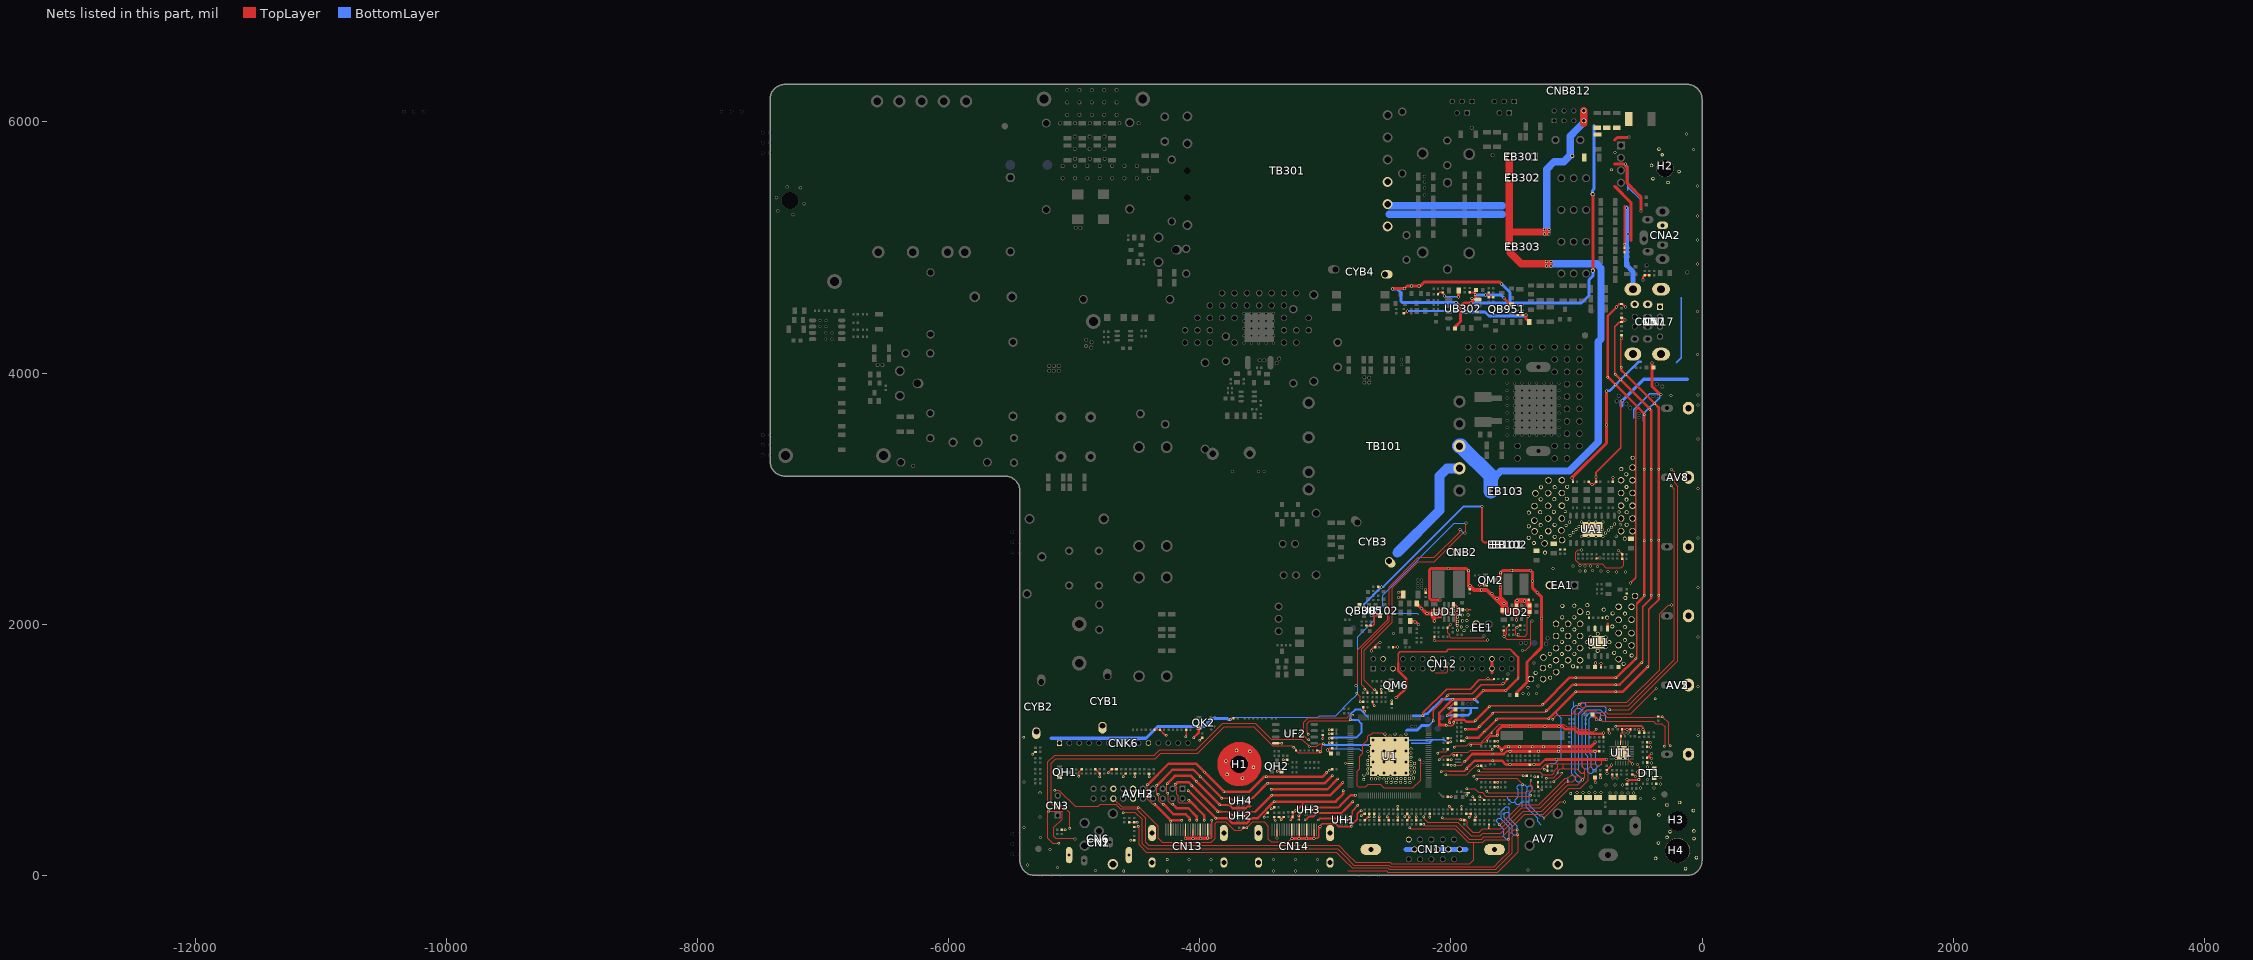
[diagram p0: the nets of this part, all layers, seen from the top]
# Altium PCB MISC84277.PcbDoc (part 9 of 15)
Units mil, origin at the board's own origin, x right, y up, seen from the top; angles counter-clockwise.
Board outline 7422.08 x 6299.21 mil, 2 copper layers (TopLayer, BottomLayer), stack 61.855 mil thick; 709 components, 395 nets, 2812 pads, 811 vias.

## Via types
v1: diameter 23.62, hole 15.75, TopLayer to BottomLayer, tented both sides, 437 vias
v2: diameter 19.68, hole 11.81, TopLayer to BottomLayer, tented both sides, 353 vias
v3: diameter 31.5, hole 23.62, TopLayer to BottomLayer, tented both sides, 16 vias
v4: diameter 31.5, hole 19.68, TopLayer to BottomLayer, tented both sides, 4 vias
v5: diameter 17.72, hole 9.84, TopLayer to BottomLayer, tented both sides, 1 vias

## Nets (pads, with @x,y where several pads share a name; then routed paths per layer and width w, separated by ;. In a path a pad name is that pad's centre, name@x,y a point inside that pad or via, vN(x,y) a via of type N, cw(c..) or ccw(c..) an arc to the next point about the centre after c; other vN are vias at no path point) (continued)
GND: (continued)
  TopLayer w11.81: RB385.1@-2675.28,1989.25 CB327.2@-2638.95,1989.25 -2622.95,1989.25 -2612.2,2000 -2612.2,2070.24 ; CB323.1@-2103.27,4628 -2089.06,4642.21 RB345.2@-2065.5,4642.27 ; RB345.2@-2065.5,4642.27 RB345.2@-2065.5,4642.27 ; RB345.2@-2062.05,4642.21 RB345.2@-2065.5,4642.27 ; v1(-2050.5,4615.5) -2050.5,4620 -2065.5,4635 RB345.2@-2065.5,4642.27 ; v1(-1806.54,4625.16) -1806.4,4625.3 CB350.1@-1806.4,4658.94 ; v1@-1725.03,4623.2 -1699.45,4623.2 ; RB357.1@-1699.45,4642.21 -1699.45,4623.2 ; RB355.2@-1662.85,4604.5 CB305.2@-1699.45,4604.5 -1699.45,4623.2 ; RB951.1@-1469.49,4463.36 CB951.2@-1430.12,4463.36 v1(-1402.21,4463.35)
  TopLayer w12: QH1.E@-5116.3,782.58 v2@-5116.3,812.98 ; v2(-4963.2,790.9) -4962.73,791.37 -4962.73,824.18 -4942.68,844.23 DH9.A@-4940.9,844.23 ; CH4.1@-4831.7,844.83 -4830.91,844.83 RH55.2@-4797.44,811.37 ; v2(-4795.5,784.6) RH55.2@-4795.5,811.37 ; v2(-4729.9,817) -4729.9,818.4 -4703.77,844.53 DH8.A@-4664.5,844.53 ; v2(-4610.8,784.1) -4610.8,790.47 DH3.A@-4590.4,810.87 ; v2@-4516.6,787 DH5.A@-4516.6,811.77 ; DH4.A@-4404.7,809.37 -4403.96,808.62 v2(-4403.96,784.67) ; CK6.1@-4360.17,1160.01 CK10.1@-4317.93,1160.01 -4317.93,1159.21 -4274.72,1116 v2(-4267.6,1116) ; CH10.1@-3652.97,378.1 v2@-3628.2,378.1 ; v2(-3488,462) -3488,476 -3465.27,498.73 CH8.1@-3458,498.73 ; v2(-3431.4,529.3) -3418.73,529.3 DH2.A@-3406.63,541.4 ; CH9.1@-3408,465.27 -3408,447 -3400,439 v2(-3400,437) ; v2(-3381.8,829.4) -3351.7,829.4 QH2.E@-3350.2,830.9 ; v2@-3336.43,920.03 v2(-3336.33,919.93) DH1.A@-3304.6,919.93 ; v2(-3253.8,1021.5) -3251.53,1021.5 -3234.13,1004.1 RO10.2@-3234.13,994.42 ; v2(-3023,1088) -3020,1091 CF2.1@-3020,1118.27 ; v1(-2983.31,1000.19) v1@-2978.81,1000.19 ; v2@-2971,1055 CF25.1@-2945.73,1055 ; v2@-2971,1091 CF8.1@-2945.73,1091 ; v2@-2971,1127 CF21.1@-2945.73,1127 ; v2(-2971,1159) -2947.73,1159 CF16.1@-2945.73,1161 ; v2(-2970.43,838.04) -2967.16,838.04 -2959.2,846 CF18.1@-2945.73,846 ; CF3.2@-2956.81,970 -2978.81,992 v1@-2978.81,1000.19 ; CF23.1@-2945.73,1012 -2967,1012 v1@-2978.81,1000.19 ; v2(-2713,475) -2696.73,491.27 CF11.1@-2688,491.27 ; v1@-2638,1794 -2615,1817 CM4.2@-2603.73,1817 -2603.73,1828.27 -2578,1854 v1(-2566,1854) ; RA1.1@-2553.73,1454 v2(-2553.73,1480.73) ; CF6.1@-2471,1366.73 v2(-2471,1392) ; RM6.2@-2461.27,1817 -2428,1817 v1(-2426,1819) ; v2(-2168,463) RF19.2@-2168,490.27 ; CD7.2@-2027.27,1972 -2027.27,1974.73 -2006,1996 v1(-2003,1996) ; CF12.1@-2025,921 v2(-1999,921) ; v2@-1977,958 CF9.1@-1951.73,958 v2@-1974.59,958 ; CF10.1@-1918.27,1071 -1893.18,1071 v2(-1893.57,1070.62) ; CF4.1@-1653.27,1028.99 v2(-1627.01,1028.99) ; CF1.1@-1653.27,1069 v2@-1628,1069 ; CD12.2@-1580,1949.27 -1580,1904 v1(-1577,1901) -1558,1920 -1558,1969.73 RD7.1@-1536.73,1991 ; v1(-813.34,2526.72) -816.29,2523.77 CA15.1@-840.99,2523.77 -814.23,2523.77 v1@-813,2525 ; v1(-787,1132) -785.27,1130.27 CF39.1@-785.27,1100 ; v1(-665.5,2587) -636.46,2557.99 -636.46,2522.72 CA9.2@-635.73,2521.99 ; CT26.1@-649.76,1112.68 -649.76,1124.68 -637.19,1137.25 -637.19,1150.41 ; CT27.2@-638.66,1162.47 v1@-596.56,1162.47 ; CT27.2@-637.19,1161 -637.19,1150.41 ; v1(-621.92,1135.33) -626.54,1135.33 -637.19,1145.98 -637.19,1150.41 ; v1(-596.62,1162.41) -596.55,1162.49 CT29.1@-569.63,1162.49 -569.63,1150.41 -587.24,1132.79 v1(-588.43,1132.79)
  TopLayer w14: -2014,830 -1895.08,830 v2(-1875.34,849.74) ; v2@-1690.74,1347.26 -1687.74,1350.26 -1279.09,1350.26 v2(-1267.81,1361.54) ; -1658.13,1299.26 -1249.48,1299.26 v2(-1239.34,1309.4) ; v2(-1639.24,1237.54) -1628.52,1248.26 v2(-1219.87,1248.26) -1208.17,1259.97
  TopLayer w15: v2(-4112.6,1102.8) -4108.33,1107.07 CK3.1@-4108.33,1160.01 ; v2(-4001.9,1076.5) -4000.57,1076.5 CK1.1@-3980.6,1096.47 ; v2(-3756.43,1240) -3745.44,1250.99 CK2.2@-3731.73,1250.99 ; UF2.4@-3395.54,1052 v2(-3349,1052) ; -3077.24,541.34 -2895.42,541.34 -2873.38,563.38 ; v2(-3058,440.84) -3045.5,453.34 -2912.7,453.34 ; -3055.4,497.34 -2870.12,497.34 -2846.23,521.23 ; RV13.2@-2572,439.73 v2(-2572,465) ; v2(-2507,465) -2507,464 -2496,453 RV11.1@-2496,439.73 ; RV5.1@-2423,439.73 v2(-2423,465) ; v2(-2368,465) -2350,483 CF7.1@-2350,491.27 ; RV2.1@-2350,439.73 -2350,440.11 -2333,457.11 v2(-2333,465) ; RI15.1@-2278,439.73 v2(-2278,465) ; CF13.1@-2025,625 -1998,625 v2(-1996,627) ; v2(-2017,1331) -1979,1369 CF15.2@-1961.81,1369 ; UD11.1@-1979.3,2153.47 -1967.02,2153.47 v1@-1940.43,2126.87 ; v1@-1951.7,2097.06 -1951.7,2124.16 v1(-1948.31,2127.56) -1936.25,2115.5 CD4.1@-1912.88,2115.5 -1912.62,2115.75 -1877.44,2115.75 -1842.02,2115.75 ; CD3.2@-1849.88,2278.15 v1(-1849.88,2308.66) ; DU1.A@-1808,439.73 -1808,458 v2(-1801,465) ; RV8.2@-1653.27,740 v2(-1628,740) ; v1@-1476.7,2026.35 -1476.7,2053.35 ; v1@-1476.7,2032.35 -1476.7,2053.35 ; -1476.7,2117.85 -1476.7,2053.35 ; v1(-1386,2060) -1372.81,2073.19 CD15.1@-1372.81,2099 ; -1296,884.53 -1288.19,884.53 -1249.74,922.98 -1247.1,922.98 ; v1(-1037,3166) -1028.73,3157.73 CA25.2@-1028.73,3134 ; CA16.1@-903.27,3134.01 v1@-880.25,3111 ; v1(-876,3111) v1@-880.25,3111 ; v1@-846,989.26 -845.85,989.41 CT1.1@-818.85,989.41 CT1.1@-827.15,989.41 ; CT5.1@-809.75,804.25 -809.75,779.01 v1(-808.13,777.39) ; v1(-757.25,810.54) -758.25,810.54 -759.1,811.39 CT18.1@-759.1,839.25 -756.18,839.25 -721.97,873.46 v1(-721.97,877.36) ; CT30.1@-745.73,1163 -745.73,1139.73 v1(-738,1132) ; CT12.2@-715.97,803.63 -715.97,782.76 v1(-710.12,776.91) ; CA10.2@-711.27,3134.01 -711.27,3167.73 v1(-711,3168) ; v2(-689.29,1186.42) -686.95,1188.76 -480.4,1188.76 -471.26,1179.62 v1(-471.26,1163.26) -471,1163.52 -471,1164 -460.97,1153.97 CT7.1@-460.97,1136.59 -460.97,1152.97 ; CT11.1@-679.97,803.63 -679.97,777.36 v1(-679.47,776.86) ; v1(-632.11,3783.61) -647.5,3768.22 -647.5,3405.07 -843.73,3208.84 CA17.2@-843.73,3134 -866.73,3111 v1@-880.25,3111 ; LT11.2@-598,725.38 -598,736.02 -574.4,759.62 -498.36,759.62 -498.22,759.76 -498.22,788.5 -500.31,790.59 -500.31,863.22 ; CT9.2@-557.5,802.68 -546.92,802.68 -531.5,787.26 v1(-529.5,787.26) ; v1(-506,1163) -498.92,1155.92 CT25.2@-498.92,1135.41 ; v1(-471.79,4742) -471.79,4764.26 RA9.1@-456.29,4779.76 CA60.2@-419.79,4779.76 ; CT21.2@-438.89,1022.41 v1@-411.62,1022.41 ; CT8.1@-438.89,1058.41 v1@-410.62,1058.41 ; v1(-403.62,932.41) -408.6,937.39 LT8.2@-437.98,937.39 -436.64,937.39 v1(-403.62,970.41)
  TopLayer w15.75: QB305.E@-2728.44,2148.27 -2696.32,2116.14 v1(-2690.94,2116.14) ; v1(-2633.85,2070.86) -2633.23,2070.24 UB102.A@-2565.46,2070.24 ; RB134.2@-2580.71,2298.23 v1(-2553.06,2298.23) ; CB340.2@-2375.5,4476.77 -2364.73,4476.77 v1(-2346,4495.5) ; pad.VIA5@-2368.11,4671.26 -2349.5,4689.87 pad.VIA5@-2243.73,4689.87 ; RB352.2@-1850.5,4643.77 -1808.63,4643.77 ; v1(-1753.94,2938.4) -1753.94,2669.29 -1737.32,2652.67 EB101.2@-1662.74,2652.67 ; v1(-1577.5,4598) -1577.5,4597 -1526.88,4546.38 QB951.E@-1517.68,4546.38
  TopLayer w16: v2@-1714.79,1073.21 -1714.79,1080.41 -1687.2,1108 -1636,1108 v2(-1630,1114) ; CT6.2@-851.63,777.57 -851.63,741.39 v1(-849,738.76) ; CA61.2@-616.95,4961.69 -616.95,5026.15 v2(-616.4,5026.7) -616.4,5329.9
  TopLayer w17: v1(-2419.29,2212.6) -2403.54,2212.6 -2379.92,2236.22 C1.1@-2379.92,2238.14 -2397.68,2255.91 -2414.9,2255.91 v1(-2417.42,2253.38) ; CD6.2@-2202.2,2250.35 v1(-2202.2,2277.35) ; v1(-805.5,1687) v1(-805.5,1687) CL43.1@-805.46,1659.01 ; v1(-681.82,4527.5) -660.09,4549.23 DU4.A@-641.5,4549.23 -634.23,4549.23 v1(-610,4525)
  TopLayer w18: v2(-3840.25,561.05) -3839.25,560.05 -3762.9,560.05 -3737.66,534.81 -3633.69,534.81 -3617.45,551.05 -3597.62,551.05
  TopLayer w20: v2(-4417.02,720.92) -4247.73,890.2 -4030.8,890.2 v2(-3807.65,667.05) -3605.84,667.05 -3489.05,783.84 v2(-3471.7,783.84) -3024.5,783.84 v2(-2988.67,819.67) ; v2(-4359.93,567.8) -4230.03,437.9 v2(-4144.2,437.9) ; v2(-4342.78,716.45) -4218.03,841.2 -4051.1,841.2 v2(-3823.95,614.05) ; v2(-4290.62,567.78) -4209.74,486.9 -4112.57,486.9 -4082.1,456.43 v2@-4082.1,443.6 ; v2(-4260.82,729.12) -4197.74,792.2 -4071.39,792.2 v2(-3840.25,561.05) ; v2(-4215.7,566.9) -4184.7,535.9 -4092.28,535.9 -4025.3,468.92 v2(-4025.3,437.9) ; v2(-4195.46,725.18) -4177.44,743.2 -4091.69,743.2 v2(-3856.54,508.05) -3835.1,508.05 ; v2(-4092.44,674.66) v2(-3872.84,455.05) -3780.94,455.05 -3740.55,414.67 -3629.01,414.67 -3588.62,455.05 -3568.5,455.05 ; v2(-4086.48,599.4) -3965.8,478.72 v2(-3965.8,437.9) ; v2(-4049.78,1095.48) -4049.78,1096.2 -4007.4,1138.58 QK2.E@-4007.4,1176.8 ; -3577.31,618.05 v2(-3460.53,734.84) -3004.21,734.84 v2(-2944.54,794.5) ; -3568.11,455.05 -3540.65,455.05 v2(-3407.87,587.84) -3246,587.84 ; -3556.95,508.05 v2(-3428.17,636.84) -3238.1,636.84 ; v2(-3432.5,685.84) -3403.1,685.84 -2983.91,685.84 v2(-2902.24,767.5) ; -3209.14,587.84 -3246,587.84 ; -3208.6,636.84 -3238.1,636.84 ; -3123.62,587.84 -3094,587.84 ; -2881.88,554.88 -2798.76,638 v1(-2762,638) ; v2(-2860.87,739.58) -2963.61,636.84 -3238.1,636.84 ; v2(-2856,672) -2856,650.05 -2918.22,587.84 -3094,587.84 ; -2854.73,512.73 v2(-2782.96,584.5) ; v1(-2437,1415) -2433.13,1415 -2354.5,1493.63 -2354.5,1563.42 -2421.15,1630.06 -2421.15,1688.46 ; CM5.1@-2325.97,2025 -2295,2025 v1(-2287,2017) -2279,2017 v1(-2259,1997) ; v2@-2040,1199 -2080.5,1199 -2093.5,1212 -2093.5,1294.34 v2(-1986.84,1401) v2(-1813.78,1401) v2(-1742.52,1472.26) v2(-1562.24,1472.26) -1465.76,1568.74 -1465.76,1736.76 -1500,1771 ; v2(-2031,1270) -1980,1321 CF5.2@-1962.81,1321 ; v1@-2025.48,1683.19 v1(-2025.31,1683.35) ; v2(-2010,1216) -2012,1218 -2012,1238 -1977,1273 CF22.2@-1962.81,1273 ; v2(-1979,1220) -1979,1227.15 -1966.8,1239.34 -1944,1239.34 ; -1955,1239.34 -1944,1239.34 ; v2(-1889.11,908.09) -1830.7,966.5 -1742,966.5 ; v2(-1887,1162) -1795.39,1162 v2(-1667.13,1290.26) ; v2(-1876,1096.5) -1780.28,1096.5 v2(-1639.24,1237.54) ; v2(-1875.34,849.74) -1810.58,914.5 -1613,914.5 ; v2@-1798.66,1239.34 -1785,1253 ; -1759,966.5 -1742,966.5 ; v2@-1690.74,1347.26 -1785,1253 ; -1602,914.5 -1613,914.5 ; -1550,884.53 -1564.53,884.53 -1594.5,914.5 -1613,914.5 ; v1(-1530.21,988.47) -1557.53,988.47 -1579.5,966.5 -1742,966.5 ; v2(-1267.81,1361.54) -1054.51,1574.84 -680.94,1574.84 v2@-523.74,1732.04 ; v2(-1239.34,1309.4) -1030.9,1517.84 -657.33,1517.84 v2@-477.59,1697.59 ; -1208.17,1259.97 v2(-1007.29,1460.84) -633.72,1460.84 v2@-427.74,1666.82 ; -1103.7,1175.1 -1093.29,1164.69 -1021.29,1164.69 -1000.45,1143.85 ; -904.3,1125.9 -922.25,1143.85 -1000.45,1143.85 ; CT2.2@-869.99,1279.9 -844.65,1254.57 v1@-844.65,1239.65 ; CL4.2@-849.25,1662.94 -849.25,1690.97 v1(-847.67,1692.56) ; v1(-787,1132) -793.1,1125.9 -982.5,1125.9 -1000.45,1143.85 ; UL1.1@-753,1965.55 -753,2004.5 ; v2(-692.5,3991.39) v2(-649.12,3948.01) v2(-415.08,3713.97) -404,3702.89 -404,2211.79 ; v1(-681.82,4527.5) -681.82,4524.67 -749.5,4456.99 v2(-749.5,3967.78) v2(-689.85,3908.13) -505.58,3723.86 -461,3679.28 -461,2222.67 -517.74,2165.94 ; v2(-644.5,4046) -644.5,4024 v2(-608.12,3987.62) v2(-376.6,3756.1) -347,3726.5 -347,2200.91 ; -3246,587.84 -3174.4,587.84 -3094,587.84 ; -1944,1239.34 -1894.41,1239.34 -1879.57,1224.5 -1813.5,1224.5 -1785,1253
  TopLayer w23.62: pad.VIA5@-2466.54,4671.26 -2463.79,4674.01 -2370.86,4674.01 -2351.06,4693.81 -2245.36,4693.81 -2215.45,4723.72 -1635.82,4723.72 ; CB302.1@-1966.69,4354.5 -1966.69,4368.31 -1923.5,4411.5 -1923.5,4532.5 -1897.65,4558.35 v1(-1842.15,4558.35) UB302.4@-1814.5,4586 ; v1(-1940,4606.17) CB326.2@-1940,4650 ; v1(-1806.54,4625.16) -1806.54,4593.96 UB302.4@-1814.5,4586 ; UB302.4@-1785.28,4586 UB302.4@-1814.5,4586 ; -1611.51,4723.72 -1635.82,4723.72 ; pad.VIA5@-1596,4709 -1610.72,4723.72 -1635.82,4723.72 ; v1(-1402.21,4463.35) -1402.22,4431.81 RB364.1@-1377.91,4407.5 ; pad.VIA5@-868.11,4816.93 pad.VIA5@-868.11,5423.23
  TopLayer w24: v1@-4113.5,294.5 v1@-3937.69,294.5 ; v1(-3267.5,295) -3090.77,295 v1@-3090.55,295.22 ; v1(-2086.7,2191.85) -2087.94,2193.08 -2157.83,2193.08 -2170.7,2205.95 -2170.7,2433.63 -2160.71,2443.62 v1@-2022.62,2443.62 ; v1@-2021,2442 v1@-2022.62,2443.62 ; -1849.88,2288 -1861,2299.12 v1(-1861,2426) -1878.62,2443.62 v1(-2021,2443.62) v1@-2022.62,2443.62 ; v1(-1772,2314) -1771.5,2314.5 QM2.E@-1724,2314.5 ; -1673.86,1610.25 CN12.26@-1673.86,1724.8 ; v2(-1630,1114) -1630,1152 -1597.74,1184.26 v1(-1139,1184.26) -1112.86,1184.26 -1103.7,1175.1 ; v2@-1627.01,1028 -1621,1028 -1597,1004 v2(-1597,995) -1567.74,1024.26 -886.34,1024.26 -849.6,1061 v1@-847,1061 ; -1620,2204.1 -1605,2219.1 v1(-1605,2410) -1587,2428 v1(-1366,2428) -1352,2414 -1352,2384 ; -1597,2185.69 v1(-1578.23,2166.93) ; -1562.53,884.53 -1296,884.53 ; v1(-1530.21,988.47) v1@-846.79,988.47 ; CF37.2@-1476.19,1436 -1476.19,1456.49 -1393.76,1538.91 -1393.76,1699.24 -1280,1813 -1280,2219.33 -1352,2291.33 -1352,2384 ; -1352,2407.43 -1352,2384 ; -1247.1,922.98 v1(-762.72,922.98) ; v1(-1037,3166) -761,3442 v1(-761,3586) v1(-761,3857.5) ; -696,5487 -566.5,5357.5 -566.5,5054.8 ; -696,5664.75 -626,5664.75 -597,5635.75 -597,5621 ; -696,5856.1 -675.3,5876.8 -599.7,5876.8 ; -597,5576.8 -597,5621 ; -594,5510 -519.1,5435.1 ; -544.2,5460.2 -519.1,5435.1 ; v1@-487.7,5303.1 -487.7,5403.7 -519.1,5435.1 ; -597,5621 -597,5513 -519.1,5435.1
  TopLayer w25: v1(-398,4079.5) -398.13,4079.37 -398.13,3893.29 v1@-334.34,3829.5
  TopLayer w30: CD1.2@-2274.2,2164.33 v1(-2236.43,2126.57) -2194.87,2085 v1(-2189.41,2085) -2136.39,2085 CD5.2@-2132.7,2081.32 v1(-2132.7,2026.3) ; v1(-2087.7,2065.25) pad.VIA5@-2087.7,2097.06 ; v1@-1849.1,2307.15 -1815.5,2273.55 -1715.62,2273.55 -1589.73,2147.66 -1589.73,2097.64 -1583.9,2091.81 v1@-1506.47,2091.81 ; -1646.17,2204.1 -1620,2204.1 ; -1578.23,2092.13 -1578.23,2130.16 ; v1(-1578.23,2166.93) -1578.23,2130.16 ; UD2.2@-1476.7,2149.52 -1476.7,2131.07 -1494.01,2113.77 -1537.19,2113.77 -1561.7,2138.28 -1561.7,2170.49 -1595.31,2204.1 -1620,2204.1 ; -1620,2204.1 -1603.59,2204.1 -1578.23,2178.74 -1578.23,2130.16
  TopLayer w40: -1476.61,2117.75 -1476.7,2117.85 UD2.2@-1476.7,2149.52 -1476.7,2180.85 -1466.7,2190.85 -1408.85,2190.85 -1374.81,2156.81 CD15.1@-1374.81,2099
  TopLayer w59.06: EB303.2@-1535.57,5012.39 EB301.2@-1535.57,5721.67 ; -1531.79,5123.87 -1238.34,5123.87 ; EB303.2@-1528.48,5005.3 -1528.48,4957.61 -1440.94,4870.08 -1216.54,4870.08 ; CNB812.7@-942.06,5990.49 CNB812.8@-942.06,6088.35
  TopLayer w118.11: -3568.29,885.98 ccw(c-3685.04,885.98) -3568.29,885.98
  BottomLayer w5: -2964.5,1009.5 -2731.5,1009.5 -2715.8,993.8
  BottomLayer w6: v2(-3137,1123) v2@-3136,1123 ; -2767.48,1423.55 -2743,1448.03 -2743,1865.57 -2743,1900.7 -2611.43,2032.28 -2611.43,2084.68 -2544.09,2152.01 ; v2(-2606,1480) v2@-2604,1482 ; -2551.18,2144.92 -2544.09,2152.01 ; v2@-2519,2085 -2515.16,2088.84 -2269.84,2088.84 -2261,2080 ; v2@-2105,970 v2(-2105,973) ; v1(-1929.13,2755.91) -1899.6,2726.37 v1(-1889.76,2726.37) ; v1(-1881.89,2807.09) -1885.14,2803.83 -1972.5,2803.83 -2544.09,2232.25 -2544.09,2152.01
  BottomLayer w8: v2(-3756.43,1240) -3738.43,1258 -3061,1258 -3046,1273 -2918.03,1273 -2808.52,1382.52 ; v2(-2751,1449) -2751,1440.03 -2808.52,1382.52 ; v2@-2744,1447.03 -2808.52,1382.52 ; v2@-2329,378 v2(-2327,378) ; v2@-2217,405 v2(-2216,406) ; v2(-1920.68,443.53) v2@-1917,439.85 ; v2@-1788,870 v2@-1784,874 ; v2@-1771,627 v2(-1770.68,627.32) ; v2@-1629,701 v2(-1628,701) ; -1600.16,453 -1600.48,453.32 -1623.32,453.32 -1634.84,441.8 -1634.84,426.2 -1616,407.35 v2(-1616,404) -1579.31,367.31 -1579.31,309.31 -1557.79,287.79 v2(-1543.53,287.79) -1537.69,293.63 -1537.69,382.69 -1600.16,445.16 -1600.16,510.84 -1565.16,545.84 -1544.84,545.84 -1534,535 -1534,510 -1541,503 ; -1546,628 -1546,609.35 -1518.8,582.16 -1499.84,582.16 -1490,592 ; v2@-1470,319 v2(-1467,322) ; -1432.84,545 -1432.84,713.84 -1439.84,720.84 -1459.8,720.84 -1471,709.65 -1471,690 -1464.07,683.07 -1464.07,627.93 -1490,602 -1490,592 ; -1432.84,589 -1454.42,567.42 -1478.52,567.42 -1490,578.9 -1490,592 ; v2@-1429,718 v2(-1429,722) ; v2@-1429,720.84 -1411.84,720.84 -1392,701 ; -1285,405 -1310.49,430.49 -1310.49,453.14 -1401,543.65 -1401,666 -1392,675 -1392,701 ; v2(-1259,454) -1278,473 -1291.62,473 -1375,556.38 -1375,655.23 -1352.16,678.07 -1352.16,701.8 -1363.2,712.84 -1380.16,712.84 -1392,701 ; -1212,893 -1168,893 -1122.84,938.16 -1122.84,1251.19 -1157.84,1286.2 -1157.84,1314.16 -1139,1333 ; -1038.84,1319.1 -1038.84,1306 ; -1020.8,1381.8 -1020.8,1341.97 ; -1002.57,751.4 -1007.81,756.64 ; -959.88,1316.22 -973.26,1329.6 -996.4,1329.6 -1010.84,1315.16 -1010.84,818.67 -964.12,771.95 -946.88,771.95 -934.69,784.14 ; -954.84,872.26 -954.84,972.26 ; v1(-953,758.76) -953,765.83 -934.69,784.14 ; v1@-950.5,758.76 -951.5,759.76 -961,759.76 -976.31,744.45 -995.62,744.45 -1007.81,756.64 ; -908.81,854.76 -916.21,847.36 -938.24,847.36 ; v1(-854.5,988.47) -848.81,982.78 -848.81,884.64 -836.62,872.45 ; v2@-808.57,1242.43 -793.4,1227.26 -773.11,1227.26 -766.05,1234.32 -766.05,1276.32 -809.73,1320 -915.54,1320 -954.84,1280.7 -954.84,972.26 ; -800,890.26 -817.81,872.45 -836.62,872.45 ; -781.17,1291.44 -763.24,1309.37 -763.24,1329.34 -779.9,1346 -926.31,1346 ; -1541,503 -1562.03,503 -1574.16,490.87 -1574.16,458.16 -1511,395 -1511,333 -1500,322 -1483.35,322 -1472.16,333.2 -1472.16,362.84 v2(-1471,364) -1471,391.77 -1534,454.77 -1534,496 -1541,503 ; -1038.84,1306 -1038.84,1323.93 -1020.8,1341.97 ; -1038.84,1306 -1038.84,809.9 -1007.81,778.87 -1007.81,756.64 ; -1020.8,1341.97 -1007.17,1355.6 -973.5,1355.6 -955.46,1373.64 -935.95,1373.64 -926.2,1363.89 -926.2,1346.11 -926.31,1346 ; -954.84,972.26 -954.84,863.96 -938.24,847.36 ; -938.24,847.36 -934.69,843.8 -934.69,826.14 ; -934.69,784.14 -934.69,826.14 ; -934.69,826.14 -946.88,813.95 -964.12,813.95 -982.84,832.67 -982.84,1289.47 -926.31,1346 ; -870.62,846.95 -852.31,846.95 -836.62,862.64 -836.62,872.45 ; -870.62,846.95 -866.69,843.02 -866.69,825.64 -878.88,813.45 -896.12,813.45 -908.81,826.14 -908.81,948.3 -926.84,966.33 -926.84,1260.36 -893.2,1294 -820.5,1294 -808.5,1282 -808.5,1247.5 -806,1245 -813,1238 -843,1238 -844,1239 -844,1246.9 -858.7,1261.6 -886.2,1261.6 -898.84,1248.96 -898.84,975.1 -882.81,959.06 -882.81,859.14 -870.62,846.95
  BottomLayer w10: v2(-3162.5,441.1) v2@-3161.1,439.7 ; -2724,1324 -2720,1320 ; v2@-2686,1306 v2(-2686,1308) ; v3(-2358.3,1077.82) -2357.68,1077.2 -2184.8,1077.2 -2182.5,1079.5 -2143.7,1079.5 ; -2318.1,1050.6 -2172.6,1050.6 -2143.7,1079.5 ; -2043.4,1066.4 -2056.5,1079.5 -2143.7,1079.5 ; v2@-2001.07,1063.93 v2(-2000.3,1063.93) ; v2@-1857.91,461.09 v2(-1856,463) ; -545,3639.5 -545,3709.5 -417,3837.5 -352.44,3837.5 -339,3824.06 -339,3804.44 -467,3676.44 -467,3617 ; -207,4081 -165,4123 -165,4603.5
  BottomLayer w11: v1@-644.5,4278 v1(-641.5,4275)
  BottomLayer w11.81: v1(-2050.5,4615.5) -2041.17,4606.17 v1(-1940,4606.17) ; v1@-1806.93,4625.56 v1(-1806.54,4625.16) ; v1@-1404.96,4463.35 v1(-1402.21,4463.35)
  BottomLayer w12: v2(-4963.2,790.9) v2@-4962.2,791.9 ; v2(-4610.8,784.1) v2@-4607.8,784.1 ; v2(-4516.6,787) v2@-4514.9,787 ; v2@-4403.96,780.61 v2(-4403.96,784.67) ; v2@-3628.6,378.5 v2(-3628.2,378.1) ; v2(-3431.4,529.3) v2@-3425.41,529.3 ; v2(-3400,437) v2@-3398,437 ; v1(-2983.31,1000.19) v1@-2979.4,1004.1 ; v2@-2970.43,835.27 v2(-2970.43,838.04) ; v2@-1900.62,1070.62 v2(-1893.57,1070.62) ; -701.5,5665.3 v1(-609.1,5665.3) -593,5649.2 -593,5458.1 ; v1@-623.5,1136.91 v1(-621.92,1135.33) ; v1@-603.9,5667.8 -603.9,5665.3 v1@-603,5664.4 ; -593,5484.31 -486.8,5378.1 v1(-486.8,5291.8) ; v1(-588.43,1132.79) v1@-586.81,1134.41
  BottomLayer w14: -2357.11,1153.41 -2265.54,1153.41 -2231.75,1187.2 -2183.65,1187.2 -2173.85,1197 ; -2191.3,1197 -2173.85,1197 ; v2(-2142.8,1232.8) -2142.8,1228.05 -2173.85,1197
  BottomLayer w15: v2(-3017.7,1048) -3007.2,1037.5 -2617.9,1037.5 ; v2(-2971,1091) -2965,1097 -2753.32,1097 -2712.69,1137.63 -2712.69,1179 ; -2712.69,1198.37 -2712.69,1179 ; -2664.66,1264.66 -2720,1320 -2763,1320 -2801,1282 v2(-2801,1241) -2798.63,1238.63 -2743.28,1238.63 -2712.69,1208.04 -2712.69,1179 ; v2(-2017,1331) -2014.5,1333.5 -1787.5,1333.5 ; v1@-1952.24,2127.56 v1(-1948.31,2127.56) ; v1@-1849.88,2304.73 v1(-1849.88,2308.66)
  BottomLayer w15.75: v1(-2633.85,2070.86) -2639.63,2070.86 -2684.91,2116.14 v1(-2690.94,2116.14) -2690.94,2160.34 v1(-2553.06,2298.23) ; v1(-2346,4495.5) pad.VIA5@-1923,4495.5 ; v1(-1753.94,2938.4) -1898.21,2938.4 -2538.39,2298.23 v1@-2552.17,2298.23 ; v1(-2553.06,2298.23) v1@-2552.17,2298.23 ; v1(-2553.06,2298.23) -2553.06,2299.12 v1@-2552.17,2298.23
  BottomLayer w20: -2347,1159.19 -2269.21,1159.19 -2231.4,1197 -2191.3,1197 ; -2301.96,1272.16 -2217.24,1272.16 -2201.5,1287.9 -2186.6,1287.9 -2073.5,1401 -2059,1401 ; -2071.4,1401 -2059,1401 ; v2(-2031,1270) -2027.5,1273.5 -1864.61,1273.5 -1840.5,1297.61 -1840.5,1328.5 -1843,1331 ; -1786.2,1377.1 -1810.1,1401 -2059,1401 ; v1@-850.23,1692.56 v1(-847.67,1692.56) ; v1(-761,3857.5) -738.24,3857.5 v2(-608.12,3987.62) -507.16,4088.58 -490.16,4088.58
  BottomLayer w23.62: pad.VIA5@-2466.54,4671.26 -2427.17,4671.26 -2397.64,4641.73 -2397.64,4570.87 -2388.27,4561.5 -2157.48,4561.5 ; -2184,4561.5 -2157.48,4561.5 ; v1(-1842.15,4558.35) -1530.5,4558.35 ; v1@-1804.57,4623.2 v1(-1725.04,4623.2) -1602.7,4623.2 v1(-1577.5,4598) ; pad.VIA5@-1596,4709 -1530.5,4643.5 -1530.5,4558.35 ; v1(-1402.21,4463.35) -1410.18,4455.38 -1696.88,4455.38 -1728.6,4487.1 -1914.6,4487.1 pad.VIA5@-1923,4495.5 -1923,4526 pad.VIA5@-1958.5,4561.5 -2157.48,4561.5 ; pad.VIA5@-872.05,5425.2 -872.05,5454.72 -862.2,5464.57 -862.2,5971.7 ; pad.VIA5@-870.08,4816.93 -870.08,4774.13 -901.57,4742.64 -901.57,4617.58 -960.81,4558.35 -1530.5,4558.35
  BottomLayer w24: -5185.3,1091.95 -4428.25,1091.95 -4333,1187.2 -3962.47,1187.2 -3899.32,1250.35 -3784.25,1250.35 -3776,1242.1 v2@-3759.6,1242.1
  BottomLayer w30: -640.97,3740.22 -640.97,3774.75 v1(-632.11,3783.61) -464.22,3951.5 -119.5,3951.5 ; CNA2.1@-314.96,5177.32 CNA2.1@-287.19,5177.32
  BottomLayer w40: -2356.76,206.74 CN11.10@-2290.75,206.74 ; CN11.8@-2110.43,206.74 -1882.26,206.74 ; v1(-600.18,5316.7) -600.18,4858.18 -551.18,4809.18 CN5.10@-551.18,4668.11
  BottomLayer w59.06: -2490.96,5265.75 -1589.4,5265.75 ; TB301.2@-2490.96,5332.68 -1589.4,5332.68 ; -1662.74,3160.24 -1602.63,3220.35 -1057.29,3220.35 -826.65,3450.99 -826.65,4248.16 -804.99,4269.81 -804.99,4836.49 -838.58,4870.08 -1232.28,4870.08 ; -1238.34,5123.87 -1238.34,5623.87 -1179.13,5683.07 -1103.23,5683.07 -1050.32,5735.98 -1050.32,5887.38 -989.94,5947.76 -989.64,5947.76 -957.6,5979.79 -957.6,5980.1
  BottomLayer w78.74: -2427.89,2569.62 -2092.52,2905 -2092.52,3179.13 -2030.32,3241.33 TB101.8@-1932.31,3241.33
  BottomLayer w118.11: TB101.9@-1932.31,3418.5 -1921,3418.5 -1676.2,3173.7 ; EB103.2@-1683.3,3058.7 -1683.3,3160.54